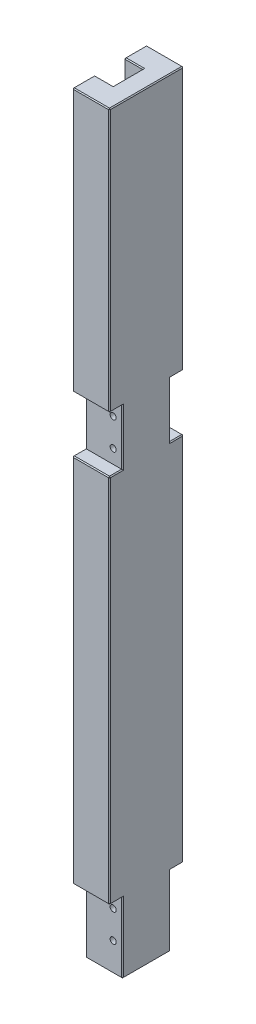
SolidWorks part; units mm, degrees
material "Al6061"
ref_plane "Front" through (0, 0, 0) normal (0, 0, 1) x (1, 0, 0)
ref_plane "Top" through (0, 0, 0) normal (0, 1, 0) x (1, 0, 0)
ref_plane "Right" through (0, 0, 0) normal (1, 0, 0) x (0, 0, -1)
sketch "草图1" plane through (0, 0, 0) normal (1, 0, 0) x (0, 0, -1)
  line L1 (-20, 205) -> (20, 205)
  line L2 (-20, 205) -> (-20, -205)
  line L3 (-20, -205) -> (20, -205)
  line L4 (20, 205) -> (20, -205)
  line L5 (-20, 205) -> (20, -205) construction
  line L6 (-20, -205) -> (20, 205) construction
  point P0 (0, 0)
  dimension "D1" = 410
  dimension "D2" = 40
extrude "凸台-拉伸1" add sketch "草图1" along normal blind 20
sketch "草图2" plane through (0, 0, 0) normal (-1, 0, 0) x (0, 0, 1)
  line L0 (20, -205) -> (-20, -205) construction
  line L1 (-8, 205) -> (8, 205)
  line L2 (-8, 205) -> (-8, -205)
  line L3 (-8, -205) -> (8, -205)
  line L4 (8, 205) -> (8, -205)
  line L5 (-8, 205) -> (8, -205) construction
  line L6 (-8, -205) -> (8, 205) construction
  point P0 (0, 0)
  dimension "D1" = 16
extrude "切除-拉伸1" cut sketch "草图2" against normal blind 10
sketch "草图3" plane through (0, 0, 20) normal (0, 0, 1) x (1, 0, 0)
  line L0 (0, 205) -> (0, -205) construction
  line L1 (0, -167) -> (20, -167)
  line L2 (0, -167) -> (0, -205)
  line L3 (0, -205) -> (20, -205)
  line L4 (20, -167) -> (20, -205)
  line L5 (20, 205) -> (20, -205) construction
  line L7 (0, 63) -> (20, 63)
  line L8 (0, 63) -> (0, 33)
  line L9 (0, 33) -> (20, 33)
  line L10 (20, 63) -> (20, 33)
  line L11 (20, -205) -> (0, -205) construction
  dimension "D1" = 38
  dimension "D2" = 30
  dimension "D3" = 200
extrude "切除-拉伸2" cut sketch "草图3" against normal blind 7
sketch "草图4" plane through (0, 0, -20) normal (0, 0, -1) x (-1, 0, 0)
  line L1 (0, 63) -> (-20, 63)
  line L2 (0, 63) -> (0, 33)
  line L3 (0, 33) -> (-20, 33)
  line L4 (-20, 63) -> (-20, 33)
  line L5 (0, -167) -> (-20, -167)
  line L6 (0, -167) -> (0, -205)
  line L7 (0, -205) -> (-20, -205)
  line L8 (-20, -167) -> (-20, -205)
extrude "切除-拉伸3" cut sketch "草图4" against normal blind 7
hole_wizard "M4 螺纹孔1" positions "草图6" profile "草图7" tap size "M4" standard "Iso" end condition through all
sketch "草图6" plane through (0, 0, -13) normal (0, 0, -1) x (-1, 0, 0)
  line L0 (-20, 48) -> (0, 48) construction
  line L1 (-20, 63) -> (-20, 33) construction
  line L2 (0, 33) -> (0, 63) construction
  line L4 (0, -167) -> (-20, -167) construction
  point P0 (-15, 55.5)
  point P2 (-15, 40.5)
  point P4 (-15, -174.4979)
  point P6 (-15, -189.4979)
  dimension "D1" = 15
  dimension "D2" = 5
  dimension "D3" = 7.4979
  dimension "D4" = 15
sketch "草图7" plane through (15, 55.5, -13) normal (1, 0, 0) x (0, 1, 0)
  line L0 (0, 0) -> (0, 33)
  line L1 (0, 33) -> (1.65, 33)
  line L2 (1.65, 33) -> (1.65, 0)
  line L5 (1.65, 0) -> (0, 0)
  line L11 (0, -6.35) -> (0, 107.95) construction
  dimension "通孔螺纹孔钻头直径" = 3.3
  dimension "通孔螺纹孔钻头深度" = 33
cosmetic thread "孔螺蚊线1" parameters "D2"=4
cosmetic thread "孔螺蚊线2" parameters "D2"=4
cosmetic thread "孔螺蚊线3" parameters "D2"=4
cosmetic thread "孔螺蚊线4" parameters "D2"=4
chamfer "倒角1" distance 0.5 angle 45 52 edges at (5, -205, -8) (10, -205, 0) (5, -205, 8) (10, -205, 13) (10, -205, -13) (0, 33, 16.5) (0, -67, 20) (0, -167, 16.5) (0, -186, 13) (0, -205, 10.5) (0, 0, 8) (0, 134, 20) (0, 48, 13) (0, 63, 16.5) (0, 33, -16.5) (0, 48, -13) (0, 63, -16.5) (0, 134, -20) (0, 0, -8) (0, -205, -10.5) (0, -186, -13) (0, -167, -16.5) (0, -67, -20) (5, 205, -8) (0, 205, -14) (10, 205, -20) (10, 205, 0) (5, 205, 8) (0, 205, 14) (10, 205, 20) (20, -186, -13) (20, -205, 0) (20, -186, 13) (20, -167, 16.5) (10, -167, 20) (20, -67, 20) (10, 33, 20) (20, 33, 16.5) (20, 48, 13) (20, 63, 16.5) (10, 63, 20) (20, 134, 20) (20, 205, 0) (20, 134, -20) (10, 63, -20) (20, 63, -16.5) (20, 48, -13) (20, 33, -16.5) (10, 33, -20) (20, -67, -20) (20, -167, -16.5) (10, -167, -20)
